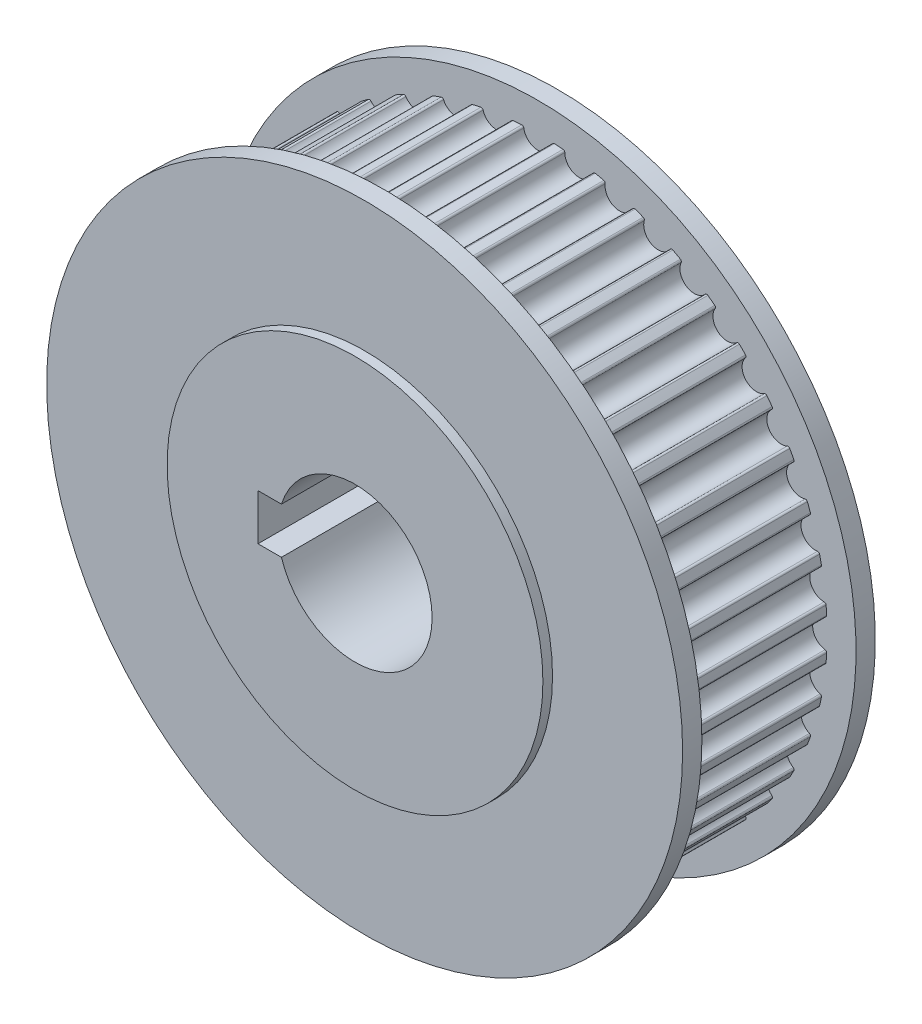
SolidWorks part; units mm, degrees
ref_plane "Front Plane" through (0, 0, 0) normal (0, 0, 1) x (1, 0, 0)
ref_plane "Top Plane" through (0, 0, 0) normal (0, 1, 0) x (1, 0, 0)
ref_plane "Right Plane" through (0, 0, 0) normal (1, 0, 0) x (0, 0, -1)
sketch "Sketch1" plane through (0, 0, 0) normal (0, 0, 1) x (1, 0, 0)
  circle A0 centre (0, 0) radius 30
  dimension "D1" = 60
extrude "Boss-Extrude1" add sketch "Sketch1" along normal blind 16
sketch "Sketch2" plane through (0, 0, 16) normal (0, 0, 1) x (1, 0, 0)
  circle A0 centre (0, 30) radius 1.5
  circle A1 centre (0, 0) radius 30 construction
  dimension "D1" = 3
extrude "Cut-Extrude1" cut sketch "Sketch2" against normal blind 16
fillet "Fillet1" radius 0.2 2 edges at (1.4995, 29.9625, 8) (-1.4995, 29.9625, 8)
pattern_circular "CirPattern1" count 44 over 360 about axis through (0, 0, 0) along (0, 0, 1) of "Cut-Extrude1", "Fillet1"
sketch "Sketch3" plane through (0, 0, 16) normal (0, 0, 1) x (1, 0, 0)
  circle A0 centre (0, 0) radius 33
  dimension "D1" = 66
extrude "Boss-Extrude2" add sketch "Sketch3" along normal blind 2
sketch "Sketch4" plane through (0, 0, 0) normal (0, 0, -1) x (-1, 0, 0)
  circle A0 centre (0, 0) radius 33
  dimension "D1" = 66
extrude "Boss-Extrude3" add sketch "Sketch4" along normal blind 2
sketch "Sketch5" plane through (0, 0, 18) normal (0, 0, 1) x (1, 0, 0)
  circle A0 centre (0, 0) radius 19.5
  dimension "D1" = 39
extrude "Boss-Extrude4" add sketch "Sketch5" along normal blind 1
sketch "Sketch6" plane through (0, 0, -2) normal (0, 0, -1) x (-1, 0, 0)
  circle A0 centre (0, 0) radius 19.5
  dimension "D1" = 39
extrude "Boss-Extrude5" add sketch "Sketch6" along normal blind 1
sketch "Sketch7" plane through (0, 0, -3) normal (0, 0, -1) x (-1, 0, 0)
  line L1 (10.0674, 2.3883) -> (7.6352, 2.3883)
  line L2 (10.0674, 2.3883) -> (10.0674, -2.3883)
  line L3 (10.0674, -2.3883) -> (7.6352, -2.3883)
  line L5 (10.0674, 2.3883) -> (8, 0) construction
  line L6 (10.0674, -2.3883) -> (8, 0) construction
  arc A0 (7.6352, 2.3883) -> (7.6352, -2.3883) centre (0, 0) ccw
  point P3 (8, 0)
  dimension "D1" = 16
extrude "Cut-Extrude2" cut sketch "Sketch7" against normal up to next
